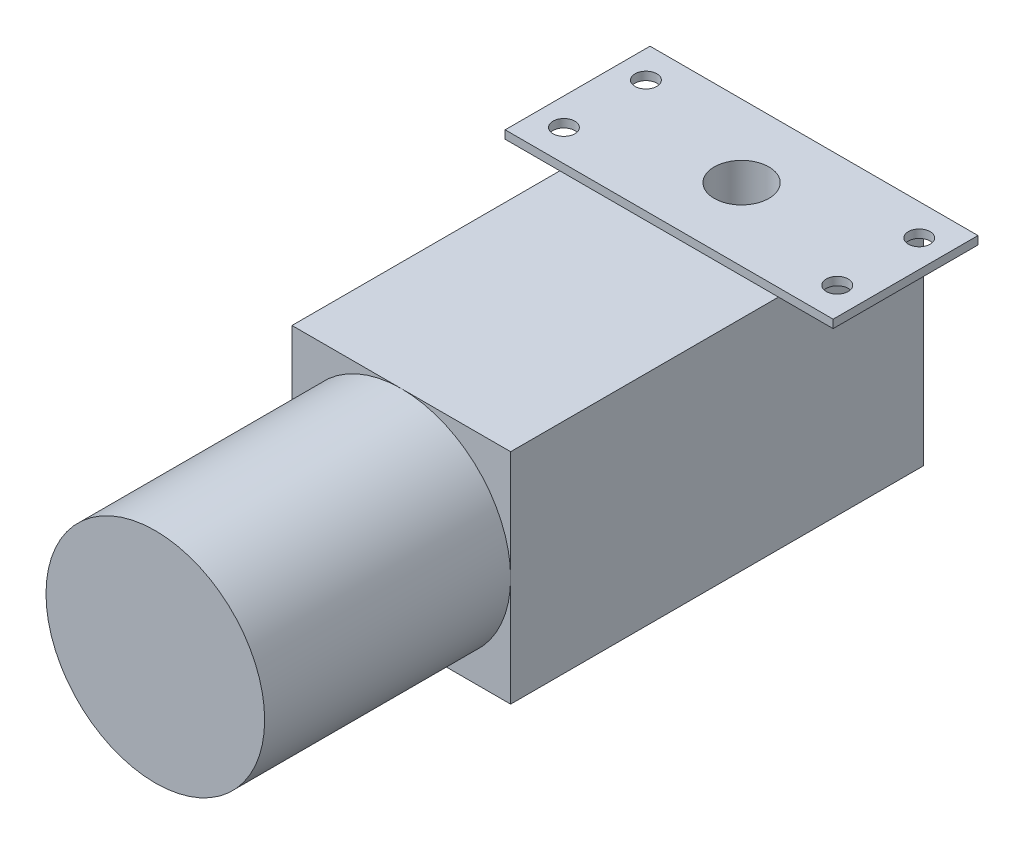
SolidWorks part; units mm, degrees
ref_plane "前视基准面" through (0, 0, 0) normal (0, 0, 1) x (1, 0, 0)
ref_plane "上视基准面" through (0, 0, 0) normal (0, 1, 0) x (1, 0, 0)
ref_plane "右视基准面" through (0, 0, 0) normal (1, 0, 0) x (0, 0, -1)
sketch "草图1" plane through (0, 0, 0) normal (0, 0, 1) x (1, 0, 0)
  line L1 (40, 40) -> (-40, 40)
  line L2 (40, 40) -> (40, -40)
  line L3 (40, -40) -> (-40, -40)
  line L4 (-40, 40) -> (-40, -40)
  line L5 (40, 40) -> (-40, -40) construction
  line L6 (40, -40) -> (-40, 40) construction
  point P0 (0, 0)
  dimension "D1" = 80
  dimension "D2" = 80
extrude "凸台-拉伸1" add sketch "草图1" along normal blind 241
sketch "草图2" plane through (0, 40, 0) normal (0, 1, 0) x (1, 0, 0)
  line L1 (-60, 0) -> (60, 0)
  line L2 (-60, 0) -> (-60, -53)
  line L3 (-60, -53) -> (60, -53)
  line L4 (60, 0) -> (60, -53)
  line L5 (0, 15.6811) -> (0, -11.2556) construction
  line L6 (40, 0) -> (-40, 0) construction
  point P4 (0, 0)
  dimension "D1" = 120
  dimension "D2" = 53
extrude "凸台-拉伸2" add sketch "草图2" along normal blind 3
sketch "草图3" plane through (0, 43, 0) normal (0, 1, 0) x (1, 0, 0)
  line L0 (-50, -11.5) -> (50, -11.5) construction
  line L1 (50, -11.5) -> (50, -41.5) construction
  line L2 (50, -41.5) -> (-50, -41.5) construction
  line L3 (-50, -41.5) -> (-50, -11.5) construction
  line L4 (-64.8825, -26.5) -> (-55.0334, -26.5) construction
  line L6 (-60, -53) -> (60, -53) construction
  circle A0 centre (-50, -11.5) radius 4
  circle A1 centre (50, -11.5) radius 4
  circle A2 centre (50, -41.5) radius 4
  circle A3 centre (-50, -41.5) radius 4
  point P8 (0, -11.5)
  point P12 (-50, -26.5)
  dimension "D1" = 8
  dimension "D2" = 8
  dimension "D3" = 8
  dimension "D4" = 8
  dimension "D5" = 100
  dimension "D6" = 30
  dimension "D7" = 26.5
extrude "切除-拉伸1" cut sketch "草图3" against normal through all
sketch "草图4" plane through (0, 43, 0) normal (0, 1, 0) x (1, 0, 0)
  circle A0 centre (0, -26.5) radius 10
  dimension "D1" = 20
extrude "切除-拉伸2" cut sketch "草图4" against normal through all
sketch "草图5" plane through (0, 0, 241) normal (0, 0, 1) x (1, 0, 0)
  circle A0 centre (0, 0) radius 40
  dimension "D1" = 80
extrude "切除-拉伸3" cut sketch "草图5" against normal blind 90 flip side to cut
